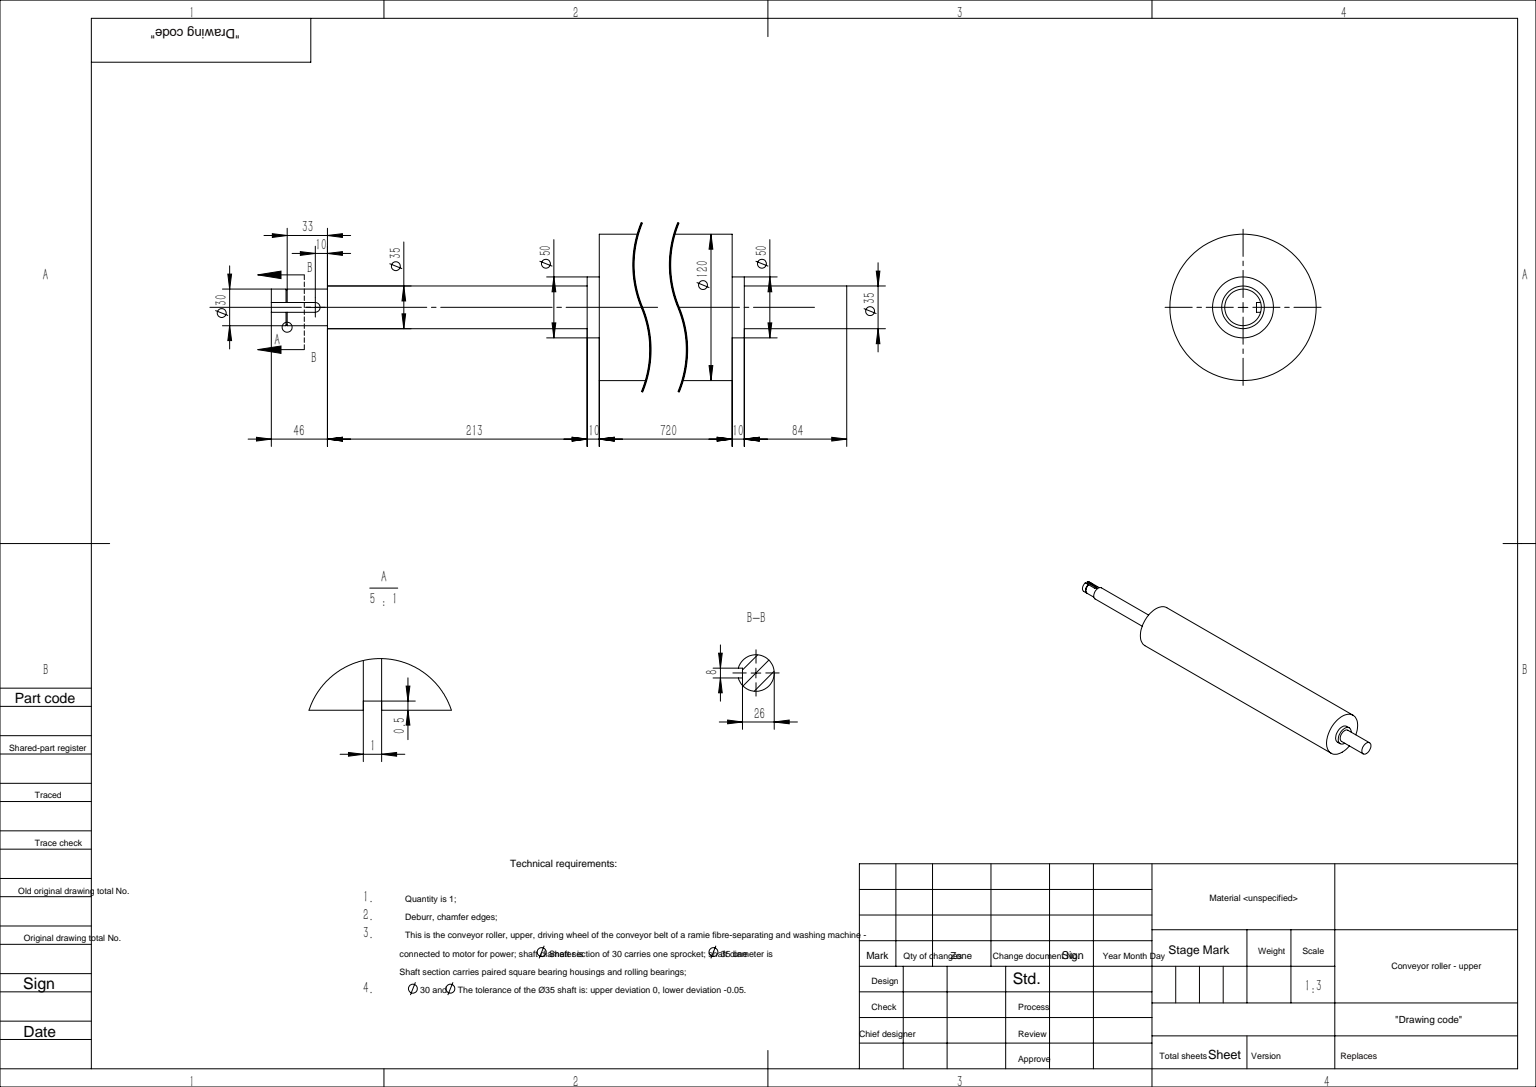
SolidWorks part; units mm, degrees
ref_plane "前视基准面" through (0, 0, 0) normal (0, 0, 1) x (1, 0, 0)
ref_plane "上视基准面" through (0, 0, 0) normal (0, 1, 0) x (1, 0, 0)
ref_plane "右视基准面" through (0, 0, 0) normal (1, 0, 0) x (0, 0, -1)
sketch "草图1" plane through (0, 0, 0) normal (0, 0, 1) x (1, 0, 0)
  line L0 (0, 0) -> (178.5616, 0) construction
  line L1 (-360, 60) -> (360, 60)
  line L2 (360, 60) -> (360, 25)
  line L3 (360, 25) -> (370, 25)
  line L4 (370, 25) -> (370, 17.5)
  line L5 (370, 17.5) -> (454, 17.5)
  line L6 (454, 17.5) -> (454, 0)
  line L7 (0, 0) -> (0, 111.0304) construction
  line L8 (-370, 25) -> (-370, 17.5)
  line L9 (-360, 25) -> (-370, 25)
  line L10 (-360, 60) -> (-360, 25)
  line L11 (-370, 17.5) -> (-583, 17.5)
  line L12 (-583, 17.5) -> (-583, 15)
  line L13 (-583, 15) -> (-629, 15)
  line L14 (-629, 15) -> (-629, 0)
  line L15 (-629, 0) -> (454, 0)
  point P15 (0, 60)
  dimension "D1" = 10
  dimension "D2" = 360
  dimension "D3" = 60
  dimension "D4" = 25
  dimension "D5" = 17.5
  dimension "D6" = 84
  dimension "D7" = 15
  dimension "D8" = 213
  dimension "D9" = 46
revolve "旋转1" add sketch "草图1" angle 360 about L15
ref_plane "基准面1" through (0, 15, 0) normal (0, 1, 0) x (1, 0, 0)
sketch "草图2" plane through (0, 15, 0) normal (0, 1, 0) x (1, 0, 0)
  line L0 (-629, 0) -> (-549.2276, 0) construction
  line L1 (-629, 15) -> (-629, -15) construction
  line L2 (-583, 17.5) -> (-583, -17.5) construction
  line L3 (-629, 4) -> (-593, 4)
  line L4 (-629, 4) -> (-629, -4)
  line L5 (-629, -4) -> (-593, -4)
  arc A0 (-593, -4) -> (-593, 4) centre (-593, 0) ccw
  dimension "D1" = 8
  dimension "D2" = 10
extrude "切除-拉伸1" cut sketch "草图2" against normal blind 4
sketch "草图3" plane through (-583, 0, 0) normal (-1, 0, 0) x (0, 0, 1)
  circle A0 centre (0, 0) radius 15
  circle A1 centre (0, 0) radius 14.3
  dimension "D1" = 28.6
  dimension "D2" = 30
extrude "切除-拉伸2" cut sketch "草图3" against normal blind 1.3 from offset 33.2
